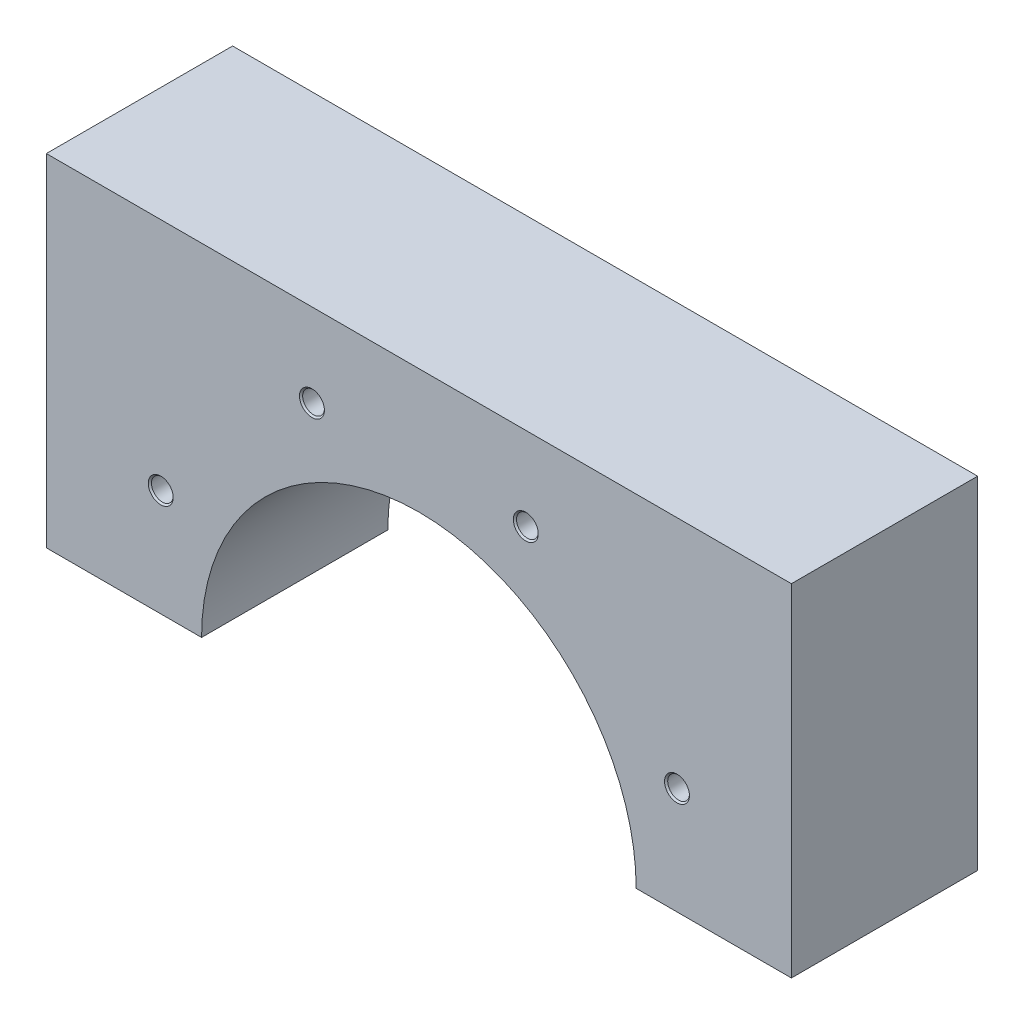
from build123d import *

# Parameters (mm, degrees)
BOSS_EXTRUDE1_DEPTH          = 120
M16_TAPPED_HOLE1_D           = 14
M16_TAPPED_HOLE1_DEPTH       = 31.793975667
M16_TAPPED_HOLE1_CSINK_D     = 16.05
M16_TAPPED_HOLE1_CSINK_ANGLE = 90
M16_TAPPED_HOLE1_TIP         = 4.206024333


with BuildPart() as part:
    # Sketch1 → Boss-Extrude1 (new body)
    with BuildSketch(Plane.XY):
        with BuildLine():
            Line((-240, 220), (240, 220))
            Line((240, 220), (240, 0))
            Line((240, 0), (140, 0))
            ThreePointArc((140, 0), (0, 140), (-140, 0))
            Line((-140, 0), (-240, 0))
            Line((-240, 0), (-240, 220))
        make_face()
    extrude(amount=BOSS_EXTRUDE1_DEPTH)

    # M16 Tapped Hole1
    with Locations(Plane.XY.offset(120)):
        with Locations((-166.298315852, 68.883017826), (-68.883017826, 166.298315852), (68.883017826, 166.298315852), (166.298315852, 68.883017826)):
            CounterSinkHole(M16_TAPPED_HOLE1_D / 2, M16_TAPPED_HOLE1_CSINK_D / 2, depth=M16_TAPPED_HOLE1_DEPTH, counter_sink_angle=M16_TAPPED_HOLE1_CSINK_ANGLE)
            with Locations((0, 0, -(M16_TAPPED_HOLE1_DEPTH + M16_TAPPED_HOLE1_TIP / 2))):  # 118° drill point
                Cone(0, M16_TAPPED_HOLE1_D / 2, M16_TAPPED_HOLE1_TIP, mode=Mode.SUBTRACT)


solid = part.part
